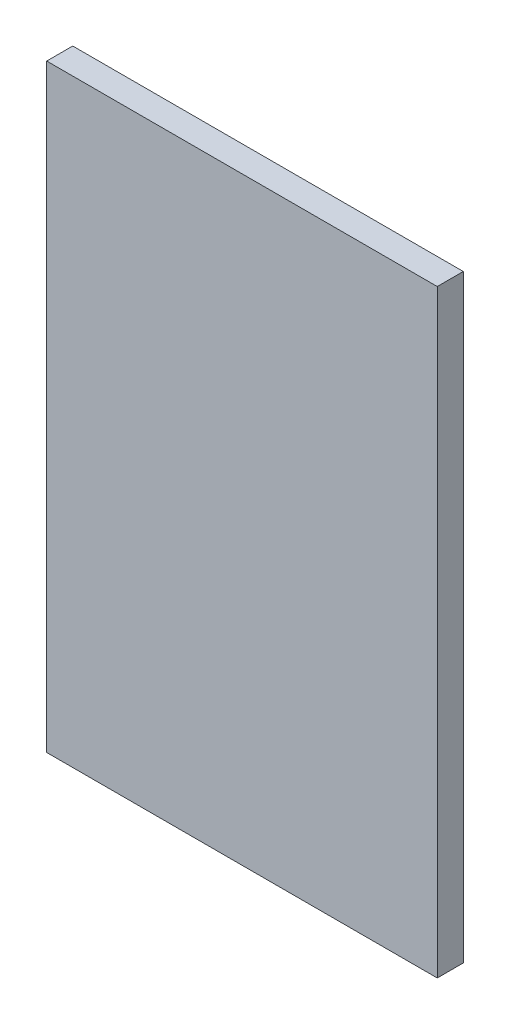
SolidWorks part; units mm, degrees
material "Q235B"
ref_plane "Front Plane" through (0, 0, 0) normal (0, 0, 1) x (1, 0, 0)
ref_plane "Top Plane" through (0, 0, 0) normal (0, 1, 0) x (1, 0, 0)
ref_plane "Right Plane" through (0, 0, 0) normal (1, 0, 0) x (0, 0, -1)
sketch "Sketch1" plane through (0, 0, 0) normal (0, 0, 1) x (1, 0, 0)
  line L1 (75, -115) -> (-75, -115)
  line L2 (75, -115) -> (75, 115)
  line L3 (75, 115) -> (-75, 115)
  line L4 (-75, -115) -> (-75, 115)
  line L5 (75, -115) -> (-75, 115) construction
  line L6 (75, 115) -> (-75, -115) construction
  point P0 (0, 0)
  dimension "D1" = 230
  dimension "D2" = 150
extrude "Boss-Extrude1" add sketch "Sketch1" along normal mid plane 10
